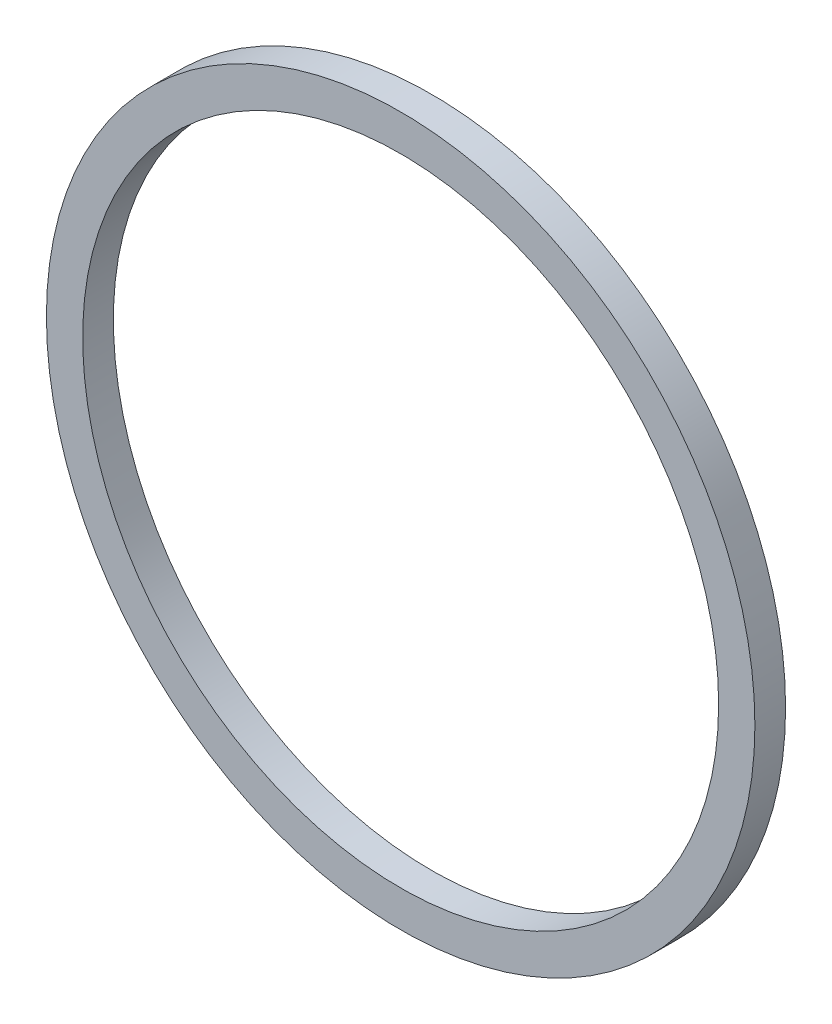
SolidWorks part; units mm, degrees
ref_plane "Front Plane" through (0, 0, 0) normal (0, 0, 1) x (1, 0, 0)
ref_plane "Top Plane" through (0, 0, 0) normal (0, 1, 0) x (1, 0, 0)
ref_plane "Right Plane" through (0, 0, 0) normal (1, 0, 0) x (0, 0, -1)
other "Configuration Table"
sketch "Sketch1" plane through (0, 0, 0) normal (0, 0, 1) x (1, 0, 0)
  circle A0 centre (0, 0) radius 63.5
  circle A1 centre (0, 0) radius 57
  dimension "D1" = 127
  dimension "D2" = 114
extrude "Boss-Extrude1" add sketch "Sketch1" along normal blind 5.5
